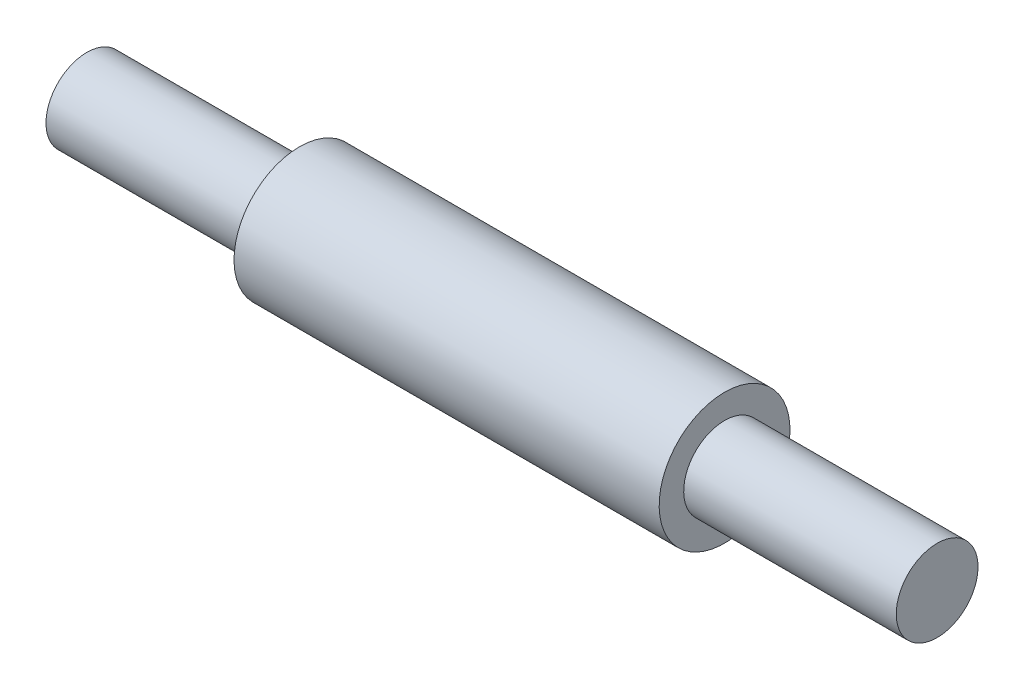
from build123d import *


with BuildPart() as part:
    # Sketch1 → Revolve1 (revolve)
    with BuildSketch(Plane.XY):
        Polygon((26, 0), (-26, 0), (-26, 2.5), (-13, 2.5), (-13, 4), (13, 4), (13, 2.5), (26, 2.5), align=None)
    revolve(axis=Axis((26, 0, 0), (-1, 0, 0)))


solid = part.part
